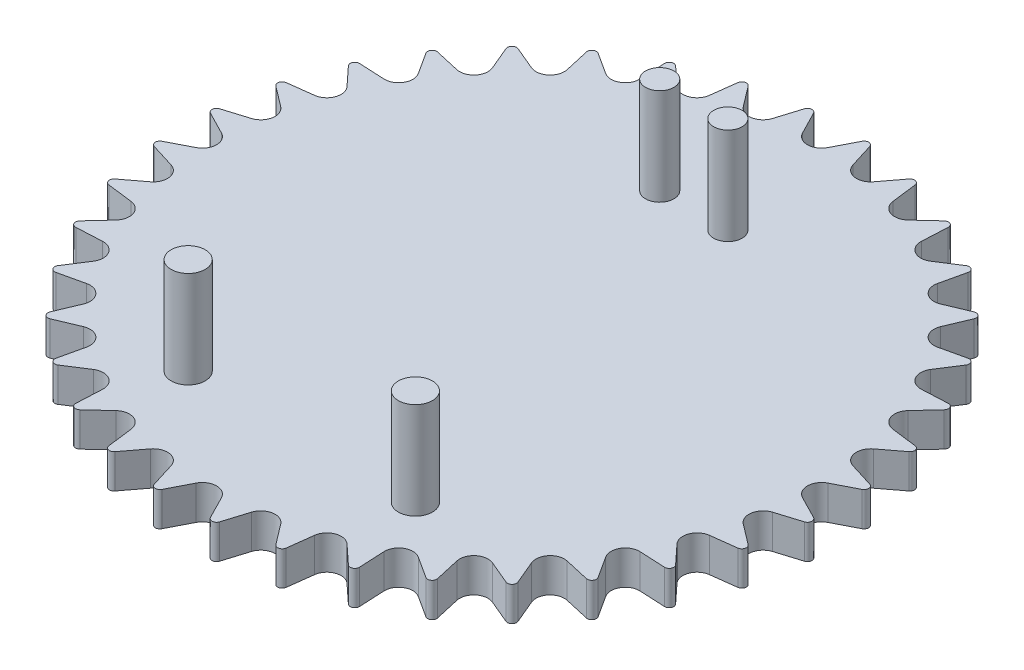
SolidWorks part; units mm, degrees
ref_plane "Front Plane" through (0, 0, 0) normal (0, 0, 1) x (1, 0, 0)
ref_plane "Top Plane" through (0, 0, 0) normal (0, 1, 0) x (1, 0, 0)
ref_plane "Right Plane" through (0, 0, 0) normal (1, 0, 0) x (0, 0, -1)
sketch "草图1" plane through (0, 0, 0) normal (0, 1, 0) x (1, 0, 0)
  circle A0 centre (0, 0) radius 290
  dimension "D1" = 580
extrude "凸台-拉伸1" add sketch "草图1" along normal blind 30
sketch "草图2" plane through (0, 30, 0) normal (0, 1, 0) x (1, 0, 0)
  line L0 (0, 290) -> (0, -290) construction
  circle A0 centre (0, 0) radius 290 construction
  circle A1 centre (-30, 160) radius 12.5
  circle A2 centre (30, 160) radius 12.5
  circle A3 centre (-100, -185) radius 15
  circle A4 centre (100, -185) radius 15
  dimension "D1" = 25
  dimension "D2" = 25
  dimension "D7" = 30
  dimension "D8" = 30
  dimension "D3" = 30
  dimension "D4" = 30
  dimension "D5" = 160
  dimension "D6" = 160
  dimension "D9" = 100
  dimension "D10" = 100
  dimension "D11" = 185
  dimension "D12" = 185
extrude "凸台-拉伸2" add sketch "草图2" along normal blind 85
ref_plane "基准面4" through (0, 15, 0) normal (0, 1, 0) x (1, 0, 0)
sketch "草图4" plane through (0, 30, 0) normal (0, 1, 0) x (1, 0, 0)
  line L0 (0, 272.5) -> (0, 0) construction
  line L1 (-25.2752, 288.8965) -> (0, 0) construction
  line L2 (0, 0) -> (25.2752, 288.8965) construction
  line L3 (-21.3686, 286.7396) -> (-11.1185, 266.7879)
  line L4 (11.1185, 266.7879) -> (21.3686, 286.7396)
  line L5 (57.2769, 260.8041) -> (70.8358, 278.6727)
  line L6 (28.7478, 286.094) -> (35.3776, 264.6655)
  line L7 (101.6948, 246.8959) -> (118.1506, 262.1385)
  line L8 (77.9908, 276.7555) -> (80.7988, 254.5014)
  line L9 (143.0229, 225.4858) -> (161.8755, 237.6394)
  line L10 (124.864, 259.008) -> (123.765, 236.6044)
  line L11 (180.0053, 197.2245) -> (200.6819, 205.9198)
  line L12 (167.9433, 233.3907) -> (162.9707, 211.5182)
  line L13 (211.5182, 162.9707) -> (233.3907, 167.9433)
  line L14 (205.9198, 200.6819) -> (197.2245, 180.0053)
  line L15 (236.6044, 123.765) -> (259.008, 124.864)
  line L16 (237.6394, 161.8755) -> (225.4858, 143.0229)
  line L17 (254.5014, 80.7988) -> (276.7555, 77.9908)
  line L18 (262.1385, 118.1506) -> (246.8959, 101.6948)
  line L19 (264.6655, 35.3776) -> (286.094, 28.7478)
  line L20 (278.6727, 70.8358) -> (260.8041, 57.2769)
  line L21 (266.7879, -11.1185) -> (286.7396, -21.3686)
  line L22 (286.7396, 21.3686) -> (266.7879, 11.1185)
  line L23 (260.8041, -57.2769) -> (278.6727, -70.8358)
  line L24 (286.094, -28.7478) -> (264.6655, -35.3776)
  line L25 (246.8959, -101.6948) -> (262.1385, -118.1506)
  line L26 (276.7555, -77.9908) -> (254.5014, -80.7988)
  line L27 (225.4858, -143.0229) -> (237.6394, -161.8755)
  line L28 (259.008, -124.864) -> (236.6044, -123.765)
  line L29 (197.2245, -180.0053) -> (205.9198, -200.6819)
  line L30 (233.3907, -167.9433) -> (211.5182, -162.9707)
  line L31 (162.9707, -211.5182) -> (167.9433, -233.3907)
  line L32 (200.6819, -205.9198) -> (180.0053, -197.2245)
  line L33 (123.765, -236.6044) -> (124.864, -259.008)
  line L34 (161.8755, -237.6394) -> (143.0229, -225.4858)
  line L35 (80.7988, -254.5014) -> (77.9908, -276.7555)
  line L36 (118.1506, -262.1385) -> (101.6948, -246.8959)
  line L37 (35.3776, -264.6655) -> (28.7478, -286.094)
  line L38 (70.8358, -278.6727) -> (57.2769, -260.8041)
  line L39 (-11.1185, -266.7879) -> (-21.3686, -286.7396)
  line L40 (21.3686, -286.7396) -> (11.1185, -266.7879)
  line L41 (-57.2769, -260.8041) -> (-70.8358, -278.6727)
  line L42 (-28.7478, -286.094) -> (-35.3776, -264.6655)
  line L43 (-101.6948, -246.8959) -> (-118.1506, -262.1385)
  line L44 (-77.9908, -276.7555) -> (-80.7988, -254.5014)
  line L45 (-143.0229, -225.4858) -> (-161.8755, -237.6394)
  line L46 (-124.864, -259.008) -> (-123.765, -236.6044)
  line L47 (-180.0053, -197.2245) -> (-200.6819, -205.9198)
  line L48 (-167.9433, -233.3907) -> (-162.9707, -211.5182)
  line L49 (-211.5182, -162.9707) -> (-233.3907, -167.9433)
  line L50 (-205.9198, -200.6819) -> (-197.2245, -180.0053)
  line L51 (-236.6044, -123.765) -> (-259.008, -124.864)
  line L52 (-237.6394, -161.8755) -> (-225.4858, -143.0229)
  line L53 (-254.5014, -80.7988) -> (-276.7555, -77.9908)
  line L54 (-262.1385, -118.1506) -> (-246.8959, -101.6948)
  line L55 (-264.6655, -35.3776) -> (-286.094, -28.7478)
  line L56 (-278.6727, -70.8358) -> (-260.8041, -57.2769)
  line L57 (-266.7879, 11.1185) -> (-286.7396, 21.3686)
  line L58 (-286.7396, -21.3686) -> (-266.7879, -11.1185)
  line L59 (-260.8041, 57.2769) -> (-278.6727, 70.8358)
  line L60 (-286.094, 28.7478) -> (-264.6655, 35.3776)
  line L61 (-246.8959, 101.6948) -> (-262.1385, 118.1506)
  line L62 (-276.7555, 77.9908) -> (-254.5014, 80.7988)
  line L63 (-225.4858, 143.0229) -> (-237.6394, 161.8755)
  line L64 (-259.008, 124.864) -> (-236.6044, 123.765)
  line L65 (-197.2245, 180.0053) -> (-205.9198, 200.6819)
  line L66 (-233.3907, 167.9433) -> (-211.5182, 162.9707)
  line L67 (-162.9707, 211.5182) -> (-167.9433, 233.3907)
  line L68 (-200.6819, 205.9198) -> (-180.0053, 197.2245)
  line L69 (-123.765, 236.6044) -> (-124.864, 259.008)
  line L70 (-161.8755, 237.6394) -> (-143.0229, 225.4858)
  line L71 (-80.7988, 254.5014) -> (-77.9908, 276.7555)
  line L72 (-118.1506, 262.1385) -> (-101.6948, 246.8959)
  line L73 (-35.3776, 264.6655) -> (-28.7478, 286.094)
  line L74 (-70.8358, 278.6727) -> (-57.2769, 260.8041)
  circle A0 centre (0, 0) radius 260 construction
  arc A1 (-11.1185, 266.7879) -> (11.1185, 266.7879) centre (0, 272.5) ccw
  circle A2 centre (0, 0) radius 290 construction
  arc A3 (-21.3686, 286.7396) -> (-25.2752, 288.8965) centre (-24.9265, 284.9117) ccw
  arc A4 (25.2752, 288.8965) -> (21.3686, 286.7396) centre (24.9265, 284.9117) ccw
  arc A6 (28.7478, 286.094) -> (25.2752, 288.8965) centre (24.9265, 284.9117) ccw
  arc A7 (75.0575, 280.1185) -> (70.8358, 278.6727) centre (74.0222, 276.2548) ccw
  arc A8 (35.3776, 264.6655) -> (57.2769, 260.8041) centre (47.3191, 268.3601) ccw
  arc A9 (77.9908, 276.7555) -> (75.0575, 280.1185) centre (74.0222, 276.2548) ccw
  arc A10 (122.5593, 262.8293) -> (118.1506, 262.1385) centre (120.8688, 259.204) ccw
  arc A11 (80.7988, 254.5014) -> (101.6948, 246.8959) centre (93.2005, 256.0662) ccw
  arc A12 (124.864, 259.008) -> (122.5593, 262.8293) centre (120.8688, 259.204) ccw
  arc A13 (166.3372, 237.5541) -> (161.8755, 237.6394) centre (164.0429, 234.2775) ccw
  arc A14 (123.765, 236.6044) -> (143.0229, 225.4858) centre (136.25, 235.9919) ccw
  arc A15 (167.9433, 233.3907) -> (166.3372, 237.5541) centre (164.0429, 234.2775) ccw
  arc A16 (205.061, 205.061) -> (200.6819, 205.9198) centre (202.2325, 202.2325) ccw
  arc A17 (162.9707, 211.5182) -> (180.0053, 197.2245) centre (175.1596, 208.7471) ccw
  arc A18 (205.9198, 200.6819) -> (205.061, 205.061) centre (202.2325, 202.2325) ccw
  arc A19 (237.5541, 166.3372) -> (233.3907, 167.9433) centre (234.2775, 164.0429) ccw
  arc A20 (197.2245, 180.0053) -> (211.5182, 162.9707) centre (208.7471, 175.1596) ccw
  arc A21 (237.6394, 161.8755) -> (237.5541, 166.3372) centre (234.2775, 164.0429) ccw
  arc A22 (262.8293, 122.5593) -> (259.008, 124.864) centre (259.204, 120.8688) ccw
  arc A23 (225.4858, 143.0229) -> (236.6044, 123.765) centre (235.9919, 136.25) ccw
  arc A24 (262.1385, 118.1506) -> (262.8293, 122.5593) centre (259.204, 120.8688) ccw
  arc A25 (280.1185, 75.0575) -> (276.7555, 77.9908) centre (276.2548, 74.0222) ccw
  arc A26 (246.8959, 101.6948) -> (254.5014, 80.7988) centre (256.0662, 93.2005) ccw
  arc A27 (278.6727, 70.8358) -> (280.1185, 75.0575) centre (276.2548, 74.0222) ccw
  arc A28 (288.8965, 25.2752) -> (286.094, 28.7478) centre (284.9117, 24.9265) ccw
  arc A29 (260.8041, 57.2769) -> (264.6655, 35.3776) centre (268.3601, 47.3191) ccw
  arc A30 (286.7396, 21.3686) -> (288.8965, 25.2752) centre (284.9117, 24.9265) ccw
  arc A31 (288.8965, -25.2752) -> (286.7396, -21.3686) centre (284.9117, -24.9265) ccw
  arc A32 (266.7879, 11.1185) -> (266.7879, -11.1185) centre (272.5, 0) ccw
  arc A33 (286.094, -28.7478) -> (288.8965, -25.2752) centre (284.9117, -24.9265) ccw
  arc A34 (280.1185, -75.0575) -> (278.6727, -70.8358) centre (276.2548, -74.0222) ccw
  arc A35 (264.6655, -35.3776) -> (260.8041, -57.2769) centre (268.3601, -47.3191) ccw
  arc A36 (276.7555, -77.9908) -> (280.1185, -75.0575) centre (276.2548, -74.0222) ccw
  arc A37 (262.8293, -122.5593) -> (262.1385, -118.1506) centre (259.204, -120.8688) ccw
  arc A38 (254.5014, -80.7988) -> (246.8959, -101.6948) centre (256.0662, -93.2005) ccw
  arc A39 (259.008, -124.864) -> (262.8293, -122.5593) centre (259.204, -120.8688) ccw
  arc A40 (237.5541, -166.3372) -> (237.6394, -161.8755) centre (234.2775, -164.0429) ccw
  arc A41 (236.6044, -123.765) -> (225.4858, -143.0229) centre (235.9919, -136.25) ccw
  arc A42 (233.3907, -167.9433) -> (237.5541, -166.3372) centre (234.2775, -164.0429) ccw
  arc A43 (205.061, -205.061) -> (205.9198, -200.6819) centre (202.2325, -202.2325) ccw
  arc A44 (211.5182, -162.9707) -> (197.2245, -180.0053) centre (208.7471, -175.1596) ccw
  arc A45 (200.6819, -205.9198) -> (205.061, -205.061) centre (202.2325, -202.2325) ccw
  arc A46 (166.3372, -237.5541) -> (167.9433, -233.3907) centre (164.0429, -234.2775) ccw
  arc A47 (180.0053, -197.2245) -> (162.9707, -211.5182) centre (175.1596, -208.7471) ccw
  arc A48 (161.8755, -237.6394) -> (166.3372, -237.5541) centre (164.0429, -234.2775) ccw
  arc A49 (122.5593, -262.8293) -> (124.864, -259.008) centre (120.8688, -259.204) ccw
  arc A50 (143.0229, -225.4858) -> (123.765, -236.6044) centre (136.25, -235.9919) ccw
  arc A51 (118.1506, -262.1385) -> (122.5593, -262.8293) centre (120.8688, -259.204) ccw
  arc A52 (75.0575, -280.1185) -> (77.9908, -276.7555) centre (74.0222, -276.2548) ccw
  arc A53 (101.6948, -246.8959) -> (80.7988, -254.5014) centre (93.2005, -256.0662) ccw
  arc A54 (70.8358, -278.6727) -> (75.0575, -280.1185) centre (74.0222, -276.2548) ccw
  arc A55 (25.2752, -288.8965) -> (28.7478, -286.094) centre (24.9265, -284.9117) ccw
  arc A56 (57.2769, -260.8041) -> (35.3776, -264.6655) centre (47.3191, -268.3601) ccw
  arc A57 (21.3686, -286.7396) -> (25.2752, -288.8965) centre (24.9265, -284.9117) ccw
  arc A58 (-25.2752, -288.8965) -> (-21.3686, -286.7396) centre (-24.9265, -284.9117) ccw
  arc A59 (11.1185, -266.7879) -> (-11.1185, -266.7879) centre (0, -272.5) ccw
  arc A60 (-28.7478, -286.094) -> (-25.2752, -288.8965) centre (-24.9265, -284.9117) ccw
  arc A61 (-75.0575, -280.1185) -> (-70.8358, -278.6727) centre (-74.0222, -276.2548) ccw
  arc A62 (-35.3776, -264.6655) -> (-57.2769, -260.8041) centre (-47.3191, -268.3601) ccw
  arc A63 (-77.9908, -276.7555) -> (-75.0575, -280.1185) centre (-74.0222, -276.2548) ccw
  arc A64 (-122.5593, -262.8293) -> (-118.1506, -262.1385) centre (-120.8688, -259.204) ccw
  arc A65 (-80.7988, -254.5014) -> (-101.6948, -246.8959) centre (-93.2005, -256.0662) ccw
  arc A66 (-124.864, -259.008) -> (-122.5593, -262.8293) centre (-120.8688, -259.204) ccw
  arc A67 (-166.3372, -237.5541) -> (-161.8755, -237.6394) centre (-164.0429, -234.2775) ccw
  arc A68 (-123.765, -236.6044) -> (-143.0229, -225.4858) centre (-136.25, -235.9919) ccw
  arc A69 (-167.9433, -233.3907) -> (-166.3372, -237.5541) centre (-164.0429, -234.2775) ccw
  arc A70 (-205.061, -205.061) -> (-200.6819, -205.9198) centre (-202.2325, -202.2325) ccw
  arc A71 (-162.9707, -211.5182) -> (-180.0053, -197.2245) centre (-175.1596, -208.7471) ccw
  arc A72 (-205.9198, -200.6819) -> (-205.061, -205.061) centre (-202.2325, -202.2325) ccw
  arc A73 (-237.5541, -166.3372) -> (-233.3907, -167.9433) centre (-234.2775, -164.0429) ccw
  arc A74 (-197.2245, -180.0053) -> (-211.5182, -162.9707) centre (-208.7471, -175.1596) ccw
  arc A75 (-237.6394, -161.8755) -> (-237.5541, -166.3372) centre (-234.2775, -164.0429) ccw
  arc A76 (-262.8293, -122.5593) -> (-259.008, -124.864) centre (-259.204, -120.8688) ccw
  arc A77 (-225.4858, -143.0229) -> (-236.6044, -123.765) centre (-235.9919, -136.25) ccw
  arc A78 (-262.1385, -118.1506) -> (-262.8293, -122.5593) centre (-259.204, -120.8688) ccw
  arc A79 (-280.1185, -75.0575) -> (-276.7555, -77.9908) centre (-276.2548, -74.0222) ccw
  arc A80 (-246.8959, -101.6948) -> (-254.5014, -80.7988) centre (-256.0662, -93.2005) ccw
  arc A81 (-278.6727, -70.8358) -> (-280.1185, -75.0575) centre (-276.2548, -74.0222) ccw
  arc A82 (-288.8965, -25.2752) -> (-286.094, -28.7478) centre (-284.9117, -24.9265) ccw
  arc A83 (-260.8041, -57.2769) -> (-264.6655, -35.3776) centre (-268.3601, -47.3191) ccw
  arc A84 (-286.7396, -21.3686) -> (-288.8965, -25.2752) centre (-284.9117, -24.9265) ccw
  arc A85 (-288.8965, 25.2752) -> (-286.7396, 21.3686) centre (-284.9117, 24.9265) ccw
  arc A86 (-266.7879, -11.1185) -> (-266.7879, 11.1185) centre (-272.5, 0) ccw
  arc A87 (-286.094, 28.7478) -> (-288.8965, 25.2752) centre (-284.9117, 24.9265) ccw
  arc A88 (-280.1185, 75.0575) -> (-278.6727, 70.8358) centre (-276.2548, 74.0222) ccw
  arc A89 (-264.6655, 35.3776) -> (-260.8041, 57.2769) centre (-268.3601, 47.3191) ccw
  arc A90 (-276.7555, 77.9908) -> (-280.1185, 75.0575) centre (-276.2548, 74.0222) ccw
  arc A91 (-262.8293, 122.5593) -> (-262.1385, 118.1506) centre (-259.204, 120.8688) ccw
  arc A92 (-254.5014, 80.7988) -> (-246.8959, 101.6948) centre (-256.0662, 93.2005) ccw
  arc A93 (-259.008, 124.864) -> (-262.8293, 122.5593) centre (-259.204, 120.8688) ccw
  arc A94 (-237.5541, 166.3372) -> (-237.6394, 161.8755) centre (-234.2775, 164.0429) ccw
  arc A95 (-236.6044, 123.765) -> (-225.4858, 143.0229) centre (-235.9919, 136.25) ccw
  arc A96 (-233.3907, 167.9433) -> (-237.5541, 166.3372) centre (-234.2775, 164.0429) ccw
  arc A97 (-205.061, 205.061) -> (-205.9198, 200.6819) centre (-202.2325, 202.2325) ccw
  arc A98 (-211.5182, 162.9707) -> (-197.2245, 180.0053) centre (-208.7471, 175.1596) ccw
  arc A99 (-200.6819, 205.9198) -> (-205.061, 205.061) centre (-202.2325, 202.2325) ccw
  arc A100 (-166.3372, 237.5541) -> (-167.9433, 233.3907) centre (-164.0429, 234.2775) ccw
  arc A101 (-180.0053, 197.2245) -> (-162.9707, 211.5182) centre (-175.1596, 208.7471) ccw
  arc A102 (-161.8755, 237.6394) -> (-166.3372, 237.5541) centre (-164.0429, 234.2775) ccw
  arc A103 (-122.5593, 262.8293) -> (-124.864, 259.008) centre (-120.8688, 259.204) ccw
  arc A104 (-143.0229, 225.4858) -> (-123.765, 236.6044) centre (-136.25, 235.9919) ccw
  arc A105 (-118.1506, 262.1385) -> (-122.5593, 262.8293) centre (-120.8688, 259.204) ccw
  arc A106 (-75.0575, 280.1185) -> (-77.9908, 276.7555) centre (-74.0222, 276.2548) ccw
  arc A107 (-101.6948, 246.8959) -> (-80.7988, 254.5014) centre (-93.2005, 256.0662) ccw
  arc A108 (-70.8358, 278.6727) -> (-75.0575, 280.1185) centre (-74.0222, 276.2548) ccw
  arc A109 (-25.2752, 288.8965) -> (-28.7478, 286.094) centre (-24.9265, 284.9117) ccw
  arc A110 (-57.2769, 260.8041) -> (-35.3776, 264.6655) centre (-47.3191, 268.3601) ccw
  circle A111 centre (0, 0) radius 330.9347
  point P331 (0, 0)
  dimension "D1" = 520
  dimension "D2" = 25
  dimension "D5" = 8
  dimension "D6" = 8
  dimension "D8" = 12.5
  dimension "D3" = 5
  dimension "D4" = 5
  dimension "D7" = 36
extrude "切除-拉伸1" cut sketch "草图4" against normal blind 30
sketch "草图5" plane through (0, 30, 0) normal (0, 1, 0) x (1, 0, 0)
  circle A0 centre (0, 0) radius 260
sketch "草图6" plane through (0, 0, 0) normal (0, -1, 0) x (1, 0, 0)
  circle A0 centre (0, 0) radius 40
  dimension "D1" = 80
extrude "Boss-Extrude3" add sketch "草图6" along normal blind 50
